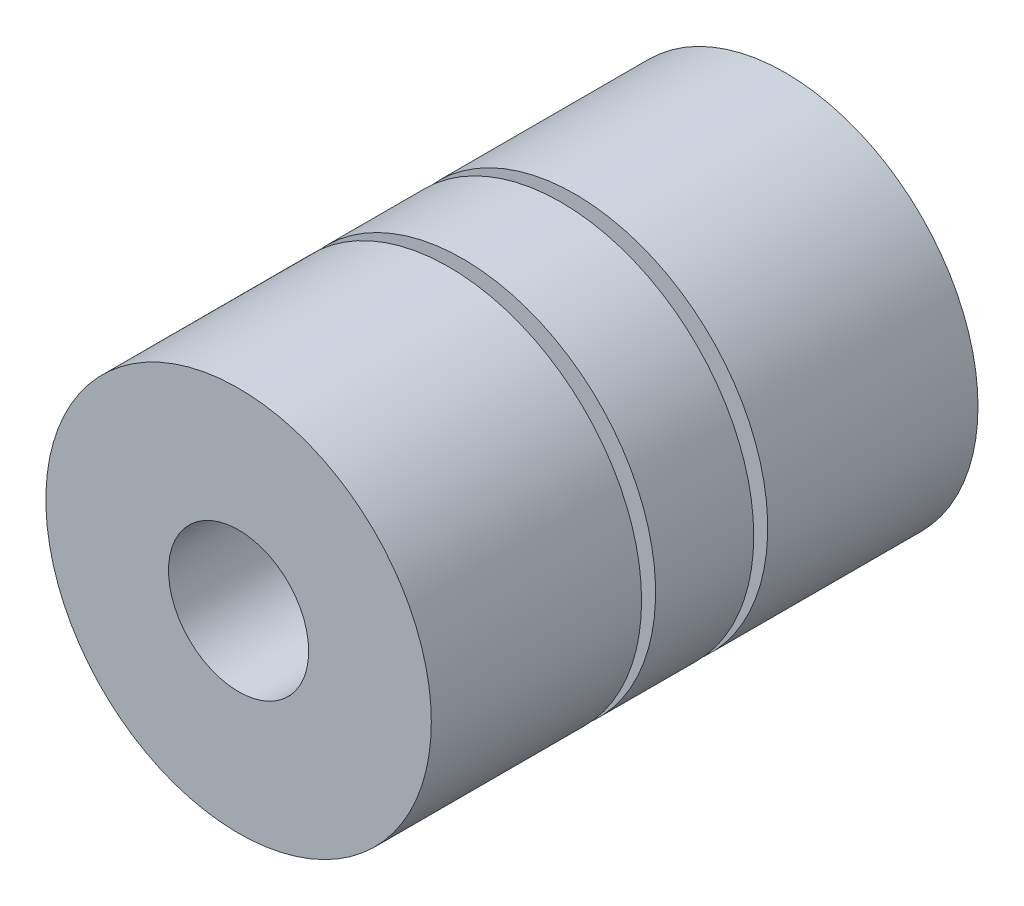
from build123d import *

# Parameters (mm, degrees)
SKETCH1_R           = 27.5
BOSS_EXTRUDE1_DEPTH = 78
SKETCH2_R           = 10
CUT_EXTRUDE1_DEPTH  = 30
SKETCH3_R           = 9.5
CUT_EXTRUDE2_DEPTH  = 30
SKETCH4_W           = 61.293657596
SKETCH4_H           = 2
CUT_EXTRUDE3_DEPTH  = 30


with BuildPart() as part:
    # Sketch1 → Boss-Extrude1 (new body)
    with BuildSketch(Plane.XY):
        Circle(SKETCH1_R)
    extrude(amount=BOSS_EXTRUDE1_DEPTH)

    # Sketch2 → Cut-Extrude1 (cut)
    with BuildSketch(Plane.XY.offset(78)):
        Circle(SKETCH2_R)
    extrude(amount=-CUT_EXTRUDE1_DEPTH, mode=Mode.SUBTRACT)

    # Sketch3 → Cut-Extrude2 (cut)
    with BuildSketch(Plane(origin=(0, 0, 0), x_dir=(-1, 0, 0), z_dir=(0, 0, -1))):
        Circle(SKETCH3_R)
    extrude(amount=-CUT_EXTRUDE2_DEPTH, mode=Mode.SUBTRACT)

    # Sketch4 → Cut-Extrude3 (cut, symmetric)
    with BuildSketch(Plane(origin=(0, 0, 0), x_dir=(1, 0, 0), z_dir=(0, 1, 0))):
        with Locations((0.888313878, -31)):
            Rectangle(SKETCH4_W, SKETCH4_H)
        with Locations((0.888313878, -47)):
            Rectangle(SKETCH4_W, SKETCH4_H)
    extrude(amount=CUT_EXTRUDE3_DEPTH, both=True, mode=Mode.SUBTRACT)


with BuildPart() as cut_extrude3_piece_1:
    # of the separate pieces the step leaves, piece 1, a body of its own (cut_extrude3_pieces)
    add(part.part.solids().sort_by_distance((27.5, 0, 0))[0])


with BuildPart() as cut_extrude3_piece_2:
    # of the separate pieces the step leaves, piece 2, a body of its own (cut_extrude3_pieces)
    add(part.part.solids().sort_by_distance((27.5, 0, 48))[0])


with BuildPart() as cut_extrude3_piece_3:
    # of the separate pieces the step leaves, piece 3, a body of its own (cut_extrude3_pieces)
    add(part.part.solids().sort_by_distance((27.5, 0, 32))[0])


solid = Compound([cut_extrude3_piece_1.part, cut_extrude3_piece_2.part, cut_extrude3_piece_3.part])
